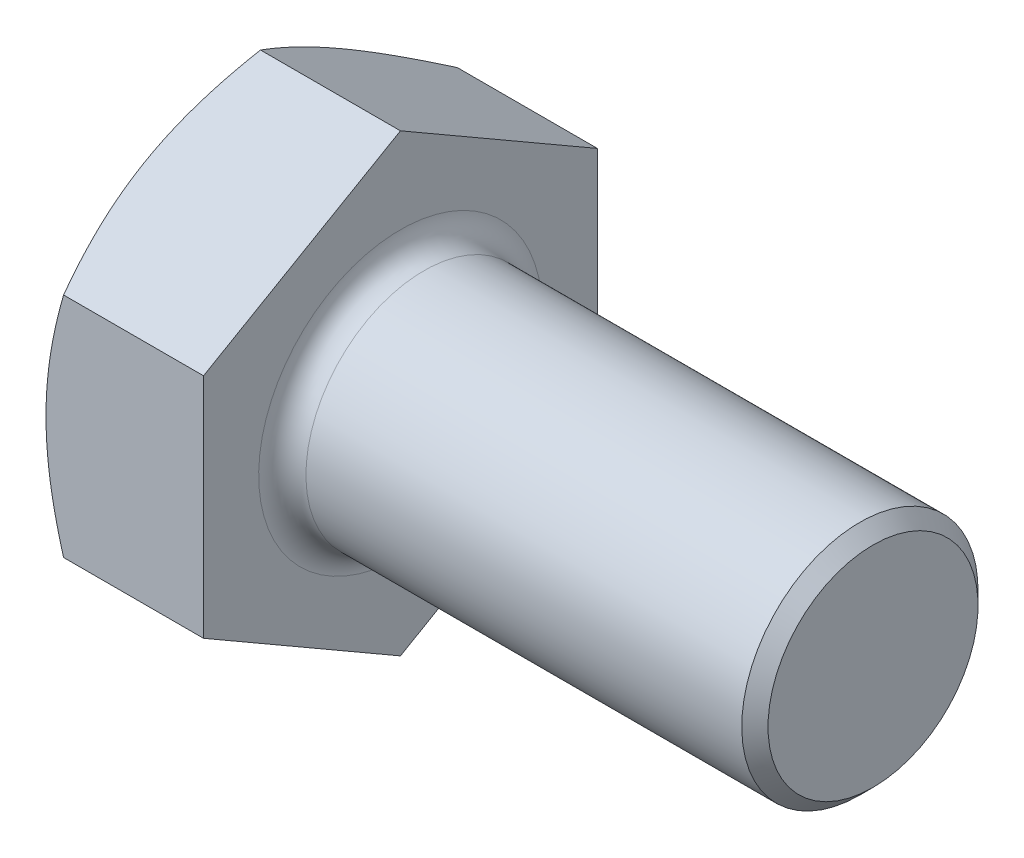
SolidWorks part; units mm, degrees
ref_plane "前视基准面" through (0, 0, 0) normal (0, 0, 1) x (1, 0, 0)
ref_plane "上视基准面" through (0, 0, 0) normal (0, 1, 0) x (1, 0, 0)
ref_plane "右视基准面" through (0, 0, 0) normal (1, 0, 0) x (0, 0, -1)
sketch "草图1" plane through (0, 0, 0) normal (0, 0, 1) x (1, 0, 0)
  line L0 (0, 0) -> (16, 0) construction
  line L1 (0, 0) -> (0, 5.445)
  line L2 (0, 5.445) -> (4, 5.445)
  line L3 (4, 5.445) -> (4, 0)
  line L4 (4, 3) -> (16, 3)
  line L5 (16, 3) -> (16, 0)
  line L6 (0, 5) -> (0.2569, 5.445)
  line L7 (14, 3) -> (14, 0)
  line L8 (7, 3) -> (7, 0)
  line L9 (4, 2.6753) -> (16, 2.6753)
  line L10 (16, 2.4588) -> (4, 2.4587)
  line L11 (3.5, 4.77) -> (4, 4.27)
  line L12 (3.5, 5.445) -> (3.5, 0)
  line L13 (3.9, 4.37) -> (3.9, 0) construction
  arc A0 (4, 3.6) -> (4.6, 3) centre (4.6, 3.6) ccw
  point P12 (15, 0)
  point P13 (1.46, 5.445)
  point P14 (4, 3.6)
  point P24 (4, 4.37)
  dimension "D1" = 0.1
  dimension "r" = 0.6
  dimension "k" = 4
  dimension "D2" = 45
  dimension "β" = 30
  dimension "e" = 10.89
  dimension "s" = 10
  dimension "d" = 6
  dimension "l" = 12
  dimension "D52" = 2
  dimension "P" = 1
  dimension "kw" = 2.54
  dimension "da" = 7.2
  dimension "a" = 3
  dimension "ds" = 5.3505
  dimension "D61" = 4.9175
  dimension "dw" = 8.74
  dimension "c" = 0.5
sketch "草图2" plane through (0, 0, 0) normal (1, 0, 0) x (0, 0, -1)
  line L1 (0, 5.7735) -> (-5, 2.8868)
  line L2 (-5, 2.8868) -> (-5, -2.8868)
  line L3 (-5, -2.8868) -> (0, -5.7735)
  line L4 (0, -5.7735) -> (5, -2.8868)
  line L5 (5, -2.8868) -> (5, 2.8868)
  line L6 (5, 2.8868) -> (0, 5.7735)
  circle A0 centre (0, 0) radius 5 construction
sketch "草图3" plane through (0, 0, 0) normal (1, 0, 0) x (0, 0, -1)
  line L0 (5, 2.8868) -> (0, 5.7735) construction
  line L1 (0, 5.7735) -> (-5, 2.8868) construction
  line L2 (-5, 2.8868) -> (-5, -2.8868) construction
  line L3 (5, -2.8868) -> (5, 2.8868) construction
  line L4 (0, -5.7735) -> (5, -2.8868) construction
  line L5 (-5, -2.8868) -> (0, -5.7735) construction
  line L6 (5, 2.8868) -> (0, 5.7735)
  line L7 (0, 5.7735) -> (-5, 2.8868)
  line L8 (-5, 2.8868) -> (-5, -2.8868)
  line L9 (5, -2.8868) -> (5, 2.8868)
  line L10 (0, -5.7735) -> (5, -2.8868)
  line L11 (-5, -2.8868) -> (0, -5.7735)
extrude "凸台-拉伸1" add sketch "草图3" along normal up to vertex (4 mm away) up to point (4, 5.445, 0)
sketch "草图4" plane through (0, 0, 0) normal (-1, 0, 0) x (0, 0, 1)
  circle A0 centre (0, 0) radius 5 construction
  circle A1 centre (0, 0) radius 5
  circle A2 centre (0, 0) radius 10.89
  dimension "D1" = 21.78
extrude "切除-拉伸1" cut sketch "草图4" against normal blind 0.5 draft 60
sketch "草图5" plane through (0, 0, 0) normal (0, 0, 1) x (1, 0, 0)
  line L0 (4, 3) -> (16, 3) construction
  line L1 (16, 3) -> (16, 0) construction
  line L2 (0, 0) -> (16, 0) construction
  line L3 (4.6, 3) -> (16, 3)
  line L4 (16, 3) -> (16, 0)
  line L5 (4, 0) -> (16, 0)
  line L6 (4, 3.6) -> (4, 0)
  arc A0 (4, 3.6) -> (4.6, 3) centre (4.6, 3.6) ccw construction
  arc A1 (4, 3.6) -> (4.6, 3) centre (4.6, 3.6) ccw
revolve "旋转1" add sketch "草图5" angle 360 about L5
cosmetic thread "装饰螺纹线2" parameters "D1"=9, "D2"=4.9175
chamfer "倒角2" distance 0.3333 angle 45 1 edges at (16, -3, 0)
sketch "草图7" plane through (0, 0, 0) normal (0, 0, 1) x (1, 0, 0)
  line L0 (4, 4.27) -> (3.5, 4.77)
  line L1 (3.5, 4.77) -> (3.5, 10.89)
  line L2 (3.5, 10.89) -> (4, 10.89)
  line L3 (4, 10.89) -> (4, 4.27)
  line L4 (0, 0) -> (16, 0) construction
  line L5 (0, 0) -> (16, 0) construction
  dimension "D1" = 21.78
revolve "切除-旋转1" [suppressed] cut sketch "草图7" angle 360 mid plane about L5
sketch "草图6" [suppressed] plane through (0, 0, 0) normal (0, 0, 1) x (1, 0, 0)
  line L0 (5.9, 0) -> (5.9, 2.5) construction
  line L1 (5.9, 2.5) -> (13.5, 2.5)
  line L2 (13.5, 2.5) -> (13.5, 0)
  line L3 (5.9, 2.5) -> (4.069, 2.245)
  line L5 (3.5, 2.2402) -> (13.5, 2.2402) construction
  line L6 (3.5, 4.315) -> (3.5, 0) construction
  line L7 (3.5, 2.7402) -> (3.5, 0)
  line L8 (3.5, 0) -> (13.5, 0)
  arc A0 (4.069, 2.245) -> (3.5, 2.7402) centre (4, 2.7402) cw
  arc A1 (3.5, 3) -> (4, 2.5) centre (4, 3) ccw construction
revolve "旋转2" add sketch "草图6" angle 360 about L8
cosmetic thread "装饰螺纹线1" [suppressed] parameters "D1"=9, "D2"=4.9175
chamfer "倒角1" [suppressed] distance 0.3333 angle 45
sketch "草图8" plane through (0, 0, 0) normal (0, 0, 1) x (1, 0, 0)
  line L0 (4, 4.27) -> (3.5, 4.77)
  line L1 (3.5, 4.77) -> (3.5, 10.89)
  line L2 (3.5, 10.89) -> (4, 10.89)
  line L3 (4, 10.89) -> (4, 4.27)
  line L4 (0, 0) -> (16, 0) construction
  line L5 (0, 0) -> (16, 0) construction
  dimension "D1" = 21.78
revolve "切除-旋转2" [suppressed] cut sketch "草图8" angle 360 mid plane about L5
